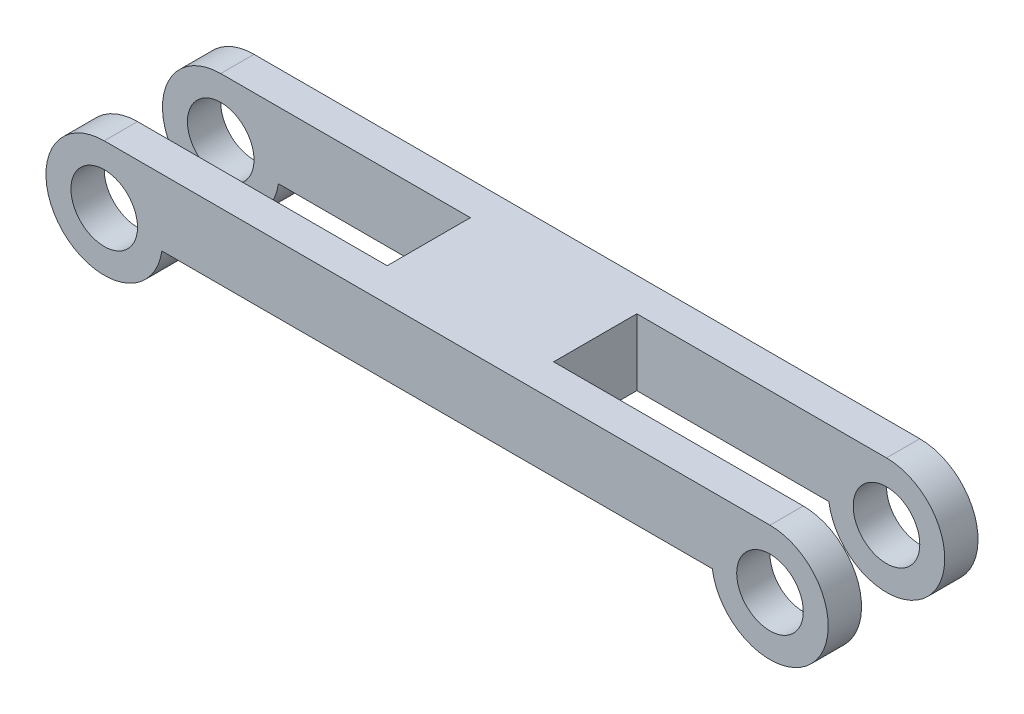
from build123d import *

# Parameters (mm, degrees)
SKETCH1_R           = 2
BOSS_EXTRUDE1_DEPTH = 9
SKETCH2_W           = 37
SKETCH2_H           = 5
CUT_EXTRUDE1_DEPTH  = 9


with BuildPart() as part:
    # Sketch1 → Boss-Extrude1 (new body)
    with BuildSketch(Plane.XY):
        with BuildLine():
            Line((-20, 0), (20, 0))
            ThreePointArc((20, 0), (22.645751311, -5.791287847), (16.535898385, -4))
            Line((16.535898385, -4), (-16.535898385, -4))
            ThreePointArc((-16.535898385, -4), (-22.645751311, -5.791287847), (-20, 0))
        make_face()
        with Locations((20, -3.5)):
            Circle(SKETCH1_R, mode=Mode.SUBTRACT)
        with Locations((-20, -3.5)):
            Circle(SKETCH1_R, mode=Mode.SUBTRACT)
    extrude(amount=BOSS_EXTRUDE1_DEPTH)

    # Sketch2 → Cut-Extrude1 (cut)
    with BuildSketch(Plane(origin=(0, 0, 0), x_dir=(1, 0, 0), z_dir=(0, 1, 0))):
        with Locations((-23.5, -4.5)):
            Rectangle(SKETCH2_W, SKETCH2_H)
    cut_extrude1 = extrude(amount=-CUT_EXTRUDE1_DEPTH, mode=Mode.SUBTRACT)

    # Mirror1: Cut-Extrude1 across plane
    add(cut_extrude1.mirror(Plane(origin=(0, 0, 0), x_dir=(0, 0, 1), z_dir=(1, 0, 0))), mode=Mode.SUBTRACT)


solid = part.part
